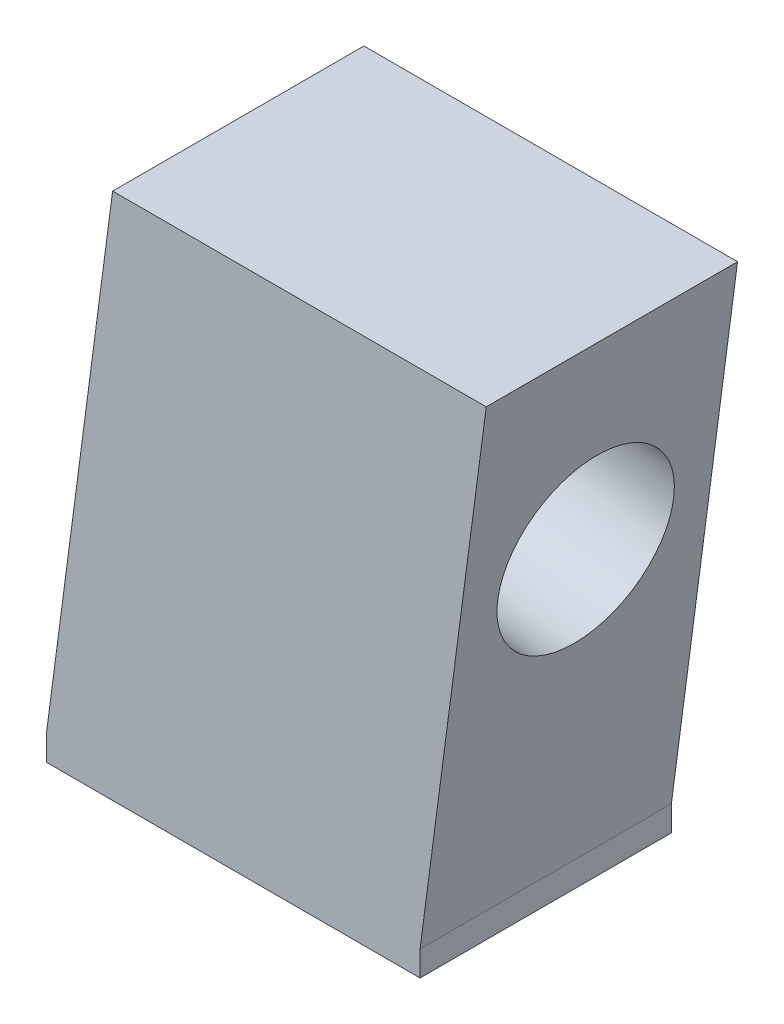
from build123d import *

# Parameters (mm, degrees)
SKETCH_1_W          = 35
SKETCH_1_H          = 42
EXTRUDE_1_DEPTH     = 20
CUT_EXTRUDE_1_REACH = 39.577
CUT_EXTRUDE_2_REACH = 47.579
SKETCH_4_R          = 7
SKETCH_5_R          = 2.1
CUT_EXTRUDE_3_DEPTH = 14
SKETCH_6_R          = 2.5
CUT_EXTRUDE_4_DEPTH = 10


with BuildPart() as part:
    # 草图1 → 凸台-拉伸1 (new body)
    with BuildSketch(Plane.XY):
        with Locations((-4.192307692, -2.269230769)):
            Rectangle(SKETCH_1_W, SKETCH_1_H)
    extrude(amount=EXTRUDE_1_DEPTH)

    # 草图3 → 切除-拉伸1 (cut, up to next)
    with BuildSketch(Plane.XY.offset(20), mode=Mode.PRIVATE) as cut_extrude_1_sk1:
        Polygon((-21.692307692, 18.730769231), (-16.426307692, 18.730769231), (-21.692307692, -21.269230769), align=None)
    cut_extrude_1_tool1 = extrude(cut_extrude_1_sk1.sketch, amount=-CUT_EXTRUDE_1_REACH, mode=Mode.PRIVATE) & part.part
    # 草图3 → 切除-拉伸1 (cut, up to next)
    with BuildSketch(Plane.XY.offset(20), mode=Mode.PRIVATE) as cut_extrude_1_sk2:
        Polygon((13.307692308, 18.730769231), (8.041692308, -21.269230769), (8.041692308, -23.269230769), (13.307692308, -23.269230769), align=None)
    cut_extrude_1_tool2 = extrude(cut_extrude_1_sk2.sketch, amount=-CUT_EXTRUDE_1_REACH, mode=Mode.PRIVATE) & part.part
    add(cut_extrude_1_tool1.solids().sort_by_distance((-19.936974, 5.397436, 20))[0], mode=Mode.SUBTRACT)
    add(cut_extrude_1_tool2.solids().sort_by_distance((11.472571, -9.238928, 20))[0], mode=Mode.SUBTRACT)

    # 草图4 → 切除-拉伸2 (cut, up to next)
    with BuildSketch(Plane(origin=(-18.570357184, 2.444787523, 0), x_dir=(0, 0, 1), z_dir=(-0.9914451818173987, 0.13052375818626055, 0)), mode=Mode.PRIVATE) as cut_extrude_2_sk1:
        with Locations(Location((10, 4.307500918, 0), (0, 0, 270))):
            Circle(SKETCH_4_R)
    cut_extrude_2_tool1 = extrude(cut_extrude_2_sk1.sketch, amount=-CUT_EXTRUDE_2_REACH, mode=Mode.PRIVATE) & part.part
    add(cut_extrude_2_tool1.solids().sort_by_distance((-18.008126, 6.715439, 10))[0], mode=Mode.SUBTRACT)

    # 草图5 → 切除-拉伸3 (cut)
    with BuildSketch(Plane.XZ.offset(23.269230769)):
        with Locations((-13.692307692, 10)):
            Circle(SKETCH_5_R)
        with Locations((0.041692308, 10)):
            Circle(SKETCH_5_R)
    extrude(amount=-CUT_EXTRUDE_3_DEPTH, mode=Mode.SUBTRACT)

    # 草图6 → 切除-拉伸4 (cut)
    with BuildSketch(Plane.XZ.offset(23.269230769)):
        with Locations((-13.692307692, 10)):
            Circle(SKETCH_6_R)
        with Locations((0.041692308, 10)):
            Circle(SKETCH_6_R)
    extrude(amount=-CUT_EXTRUDE_4_DEPTH, mode=Mode.SUBTRACT)


solid = part.part
